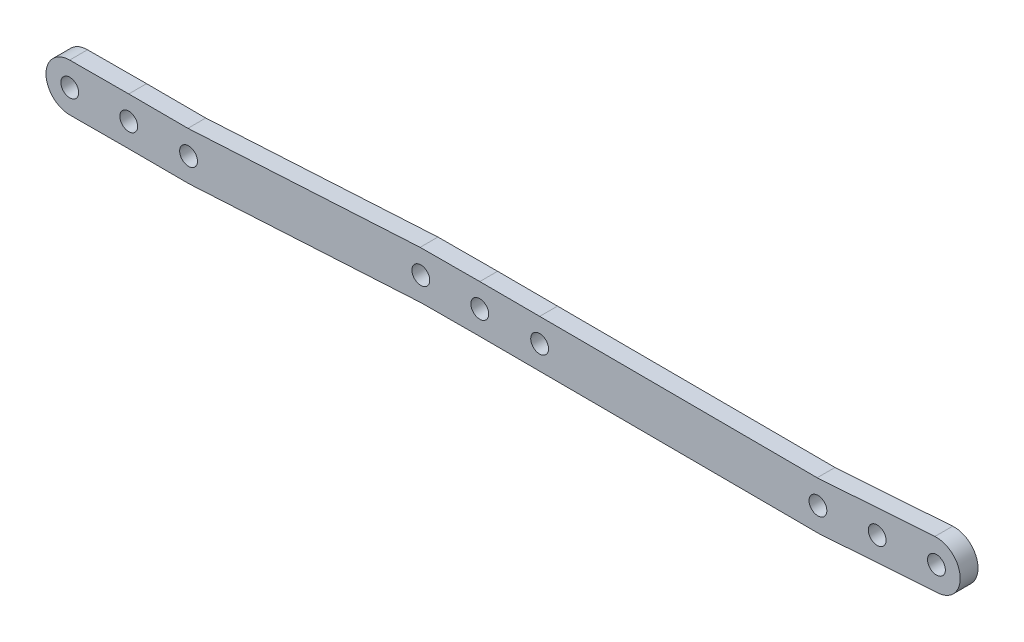
from build123d import *

# Parameters (mm, degrees)
SKETCH1_R           = 1.5
BOSS_EXTRUDE1_DEPTH = 3


with BuildPart() as part:
    # Sketch1 → Boss-Extrude1 (new body)
    with BuildSketch(Plane.XY):
        with BuildLine():
            Line((-69.019918417, -6.227312299), (-59.101906393, -6.196290568))
            Line((-59.101906393, -6.196290568), (-48.926464715, -6.227677735))
            Line((-48.926464715, -6.227677735), (-9.807058311, -4.032732904))
            Line((-9.807058311, -4.032732904), (9.82e-05, -4.000021922))
            Line((9.82e-05, -4.000021922), (10.060192173, -4.033082606))
            Line((10.060192173, -4.033082606), (57.060189179, -4.206563863))
            Line((57.060189179, -4.206563863), (67.179803064, -3.520371058))
            Line((67.179803064, -3.520371058), (77.15689228, -2.843842595))
            ThreePointArc((77.15689228, -2.843842595), (80.877116582, 1.417604476), (76.61566951, 5.137828778))
            Line((76.61566951, 5.137828778), (66.638580293, 4.461300315))
            Line((66.638580293, 4.461300315), (56.804015745, 3.794436193))
            Line((56.804015745, 3.794436193), (10.088101644, 3.966868874))
            Line((10.088101644, 3.966868874), (-9.82e-05, 4.000021922))
            Line((-9.82e-05, 4.000021922), (-10.044647872, 3.966519135))
            Line((-10.044647872, 3.966519135), (-49.138394535, 1.773014043))
            Line((-49.138394535, 1.773014043), (-59.102079262, 1.803748024))
            Line((-59.102079262, 1.803748024), (-69.044940833, 1.772648568))
            ThreePointArc((-69.044940833, 1.772648568), (-73.032410059, -2.239843074), (-69.019918417, -6.227312299))
        make_face()
        with Locations((-69.032429625, -2.227331865)):
            Circle(SKETCH1_R, mode=Mode.SUBTRACT)
        with Locations((-59.101992828, -2.196271272)):
            Circle(SKETCH1_R, mode=Mode.SUBTRACT)
        with Locations((-49.032429625, -2.227331846)):
            Circle(SKETCH1_R, mode=Mode.SUBTRACT)
        with Locations((-9.925853092, -0.033106885)):
            Circle(SKETCH1_R, mode=Mode.SUBTRACT)
        Circle(SKETCH1_R, mode=Mode.SUBTRACT)
        with Locations((10.074146909, -0.033106866)):
            Circle(SKETCH1_R, mode=Mode.SUBTRACT)
        with Locations((56.932102462, -0.206063835)):
            Circle(SKETCH1_R, mode=Mode.SUBTRACT)
        with Locations((66.909191678, 0.470464628)):
            Circle(SKETCH1_R, mode=Mode.SUBTRACT)
        with Locations((76.886280895, 1.146993091)):
            Circle(SKETCH1_R, mode=Mode.SUBTRACT)
    extrude(amount=BOSS_EXTRUDE1_DEPTH)


solid = part.part
